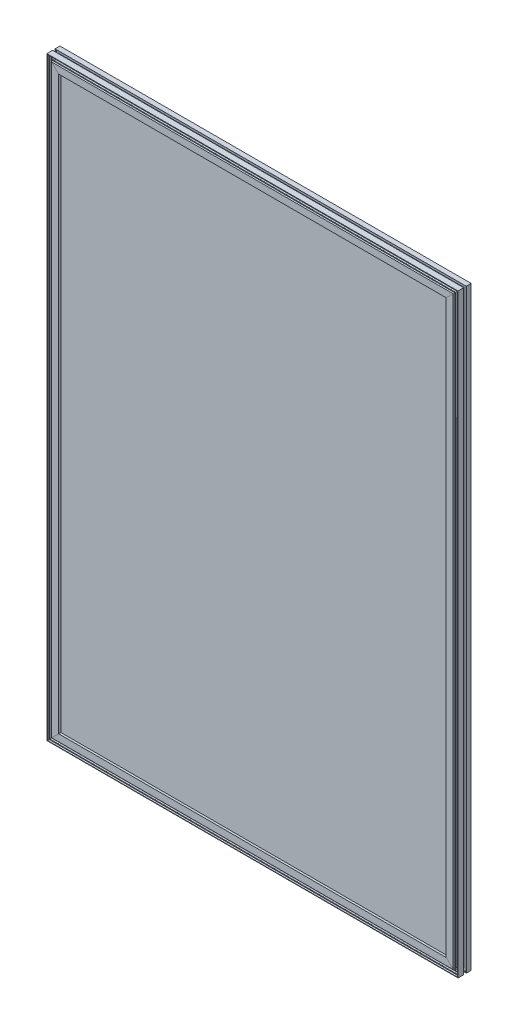
from build123d import *

# Parameters (mm, degrees)
MEMBER_250403_1_DEPTH      = 41.360872141
MEMBER_250403_1_DEPTH_BACK = 1401.360872141
MEMBER_250403_1_2_DEPTH    = 1022.721744282
MEMBER_250403_1_3_DEPTH    = 1442.721744282
MEMBER_250403_1_4_DEPTH    = 1022.721744282
SKETCH_12_W                = 900
SKETCH_12_H                = 1320
EXTRUDE_1_DEPTH            = 17


with BuildPart() as part:
    # 草图11 → Member 250403_1 (new, two sides: drawn at the far end of the back side and taken through both)
    with BuildSketch(Plane(origin=(-470, 680, 0), x_dir=(1, 0, 0), z_dir=(0, 1, 0)).offset(-MEMBER_250403_1_DEPTH_BACK)):
        with BuildLine():
            Line((11.006838108, 0), (27, 0))
            Line((27, 0), (27, 5))
            Line((27, 5), (25.5, 5))
            Line((25.5, 5), (25.5, 2.2))
            ThreePointArc((25.5, 2.2), (25.207106781, 1.492893219), (24.5, 1.2))
            Line((24.5, 1.2), (18, 1.2))
            ThreePointArc((18, 1.2), (17.292893219, 1.492893219), (17, 2.2))
            Line((17, 2.2), (17, 30))
            Line((17, 30), (12.5, 30))
            Line((12.5, 30), (12.5, 28.8))
            Line((12.5, 28.8), (15.8, 28.8))
            Line((15.8, 28.8), (15.8, 22))
            Line((15.8, 22), (1.2, 22))
            Line((1.2, 22), (1.2, 28.8))
            Line((1.2, 28.8), (4.5, 28.8))
            Line((4.5, 28.8), (4.5, 30))
            Line((4.5, 30), (0, 30))
            Line((0, 30), (0, 18.8))
            Line((0, 18.8), (1.2, 18.8))
            Line((1.2, 18.8), (1.2, 20.8))
            Line((1.2, 20.8), (6.7, 20.8))
            Line((6.7, 20.8), (6.7, 18.8))
            Line((6.7, 18.8), (7.7, 18.8))
            Line((7.7, 18.8), (7.7, 13))
            Line((7.7, 13), (6.7, 13))
            Line((6.7, 13), (6.7, 11))
            Line((6.7, 11), (1.2, 11))
            Line((1.2, 11), (1.2, 13))
            Line((1.2, 13), (0, 13))
            Line((0, 13), (0, 0))
            Line((0, 0), (1.006838108, 0))
            Line((1.006838108, 0), (2.380431303, 2.400675266))
            ThreePointArc((2.380431303, 2.400675266), (2.379848147, 2.600337065), (2.206838108, 2.7))
            Line((2.206838108, 2.7), (1.706838108, 2.7))
            Line((1.706838108, 2.7), (1.706838108, 2.9))
            Line((1.706838108, 2.9), (2.675186721, 3.252126768))
            ThreePointArc((2.675186721, 3.252126768), (2.770651604, 3.325346014), (2.806838108, 3.440085453))
            Line((2.806838108, 3.440085453), (2.806838108, 3.9))
            ThreePointArc((2.806838108, 3.9), (2.748259465, 4.041421356), (2.606838108, 4.1))
            Line((2.606838108, 4.1), (1.006838108, 4.1))
            Line((1.006838108, 4.1), (1.006838108, 9.5))
            ThreePointArc((1.006838108, 9.5), (1.153284718, 9.853553391), (1.506838108, 10))
            Line((1.506838108, 10), (10.506838108, 10))
            ThreePointArc((10.506838108, 10), (10.860391499, 9.853553391), (11.006838108, 9.5))
            Line((11.006838108, 9.5), (11.006838108, 4.1))
            Line((11.006838108, 4.1), (9.406838108, 4.1))
            ThreePointArc((9.406838108, 4.1), (9.265416752, 4.041421356), (9.206838108, 3.9))
            Line((9.206838108, 3.9), (9.206838108, 3.440085453))
            ThreePointArc((9.206838108, 3.440085453), (9.243024613, 3.325346014), (9.338489496, 3.252126768))
            Line((9.338489496, 3.252126768), (10.306838108, 2.9))
            Line((10.306838108, 2.9), (10.306838108, 2.7))
            Line((10.306838108, 2.7), (9.806838108, 2.7))
            ThreePointArc((9.806838108, 2.7), (9.63382807, 2.600337065), (9.633244913, 2.400675266))
            Line((9.633244913, 2.400675266), (11.006838108, 0))
        make_face()
        with BuildLine():
            Line((7.9, 11), (7.9, 11.8))
            ThreePointArc((7.9, 11.8), (8.607106781, 12.092893219), (8.9, 12.8))
            Line((8.9, 12.8), (8.9, 19))
            ThreePointArc((8.9, 19), (8.607106781, 19.707106781), (7.9, 20))
            Line((7.9, 20), (7.9, 20.8))
            Line((7.9, 20.8), (16, 20.8))
            Line((16, 20.8), (16, 1.2))
            Line((16, 1.2), (12.006838108, 1.2))
            Line((12.006838108, 1.2), (12.006838108, 11))
            Line((12.006838108, 11), (7.9, 11))
        make_face(mode=Mode.SUBTRACT)
    extrude(amount=MEMBER_250403_1_DEPTH + MEMBER_250403_1_DEPTH_BACK)

    # Member 250403_1 mitre 1
    split(bisect_by=Plane(origin=(-470, 680, 0), x_dir=(0.707106781, -0.707106781, 0), z_dir=(-0.707106781, -0.707106781, 0)), keep=Keep.TOP)

    # Member 250403_1 mitre 2
    split(bisect_by=Plane(origin=(-470, -680, 0), x_dir=(-0.707106781, -0.707106781, 0), z_dir=(-0.707106781, 0.707106781, 0)), keep=Keep.TOP)


with BuildPart() as body_2:
    # 草图11 on segment 2 (carried to segment 2) → Member 250403_1 2 (new body)
    with BuildSketch(Plane(origin=(511.360872141, -680, 0), x_dir=(0, 1, 0), z_dir=(-1, 0, 0))):
        with BuildLine():
            Line((11.006838108, 0), (27, 0))
            Line((27, 0), (27, 5))
            Line((27, 5), (25.5, 5))
            Line((25.5, 5), (25.5, 2.2))
            ThreePointArc((25.5, 2.2), (25.207106781, 1.492893219), (24.5, 1.2))
            Line((24.5, 1.2), (18, 1.2))
            ThreePointArc((18, 1.2), (17.292893219, 1.492893219), (17, 2.2))
            Line((17, 2.2), (17, 30))
            Line((17, 30), (12.5, 30))
            Line((12.5, 30), (12.5, 28.8))
            Line((12.5, 28.8), (15.8, 28.8))
            Line((15.8, 28.8), (15.8, 22))
            Line((15.8, 22), (1.2, 22))
            Line((1.2, 22), (1.2, 28.8))
            Line((1.2, 28.8), (4.5, 28.8))
            Line((4.5, 28.8), (4.5, 30))
            Line((4.5, 30), (0, 30))
            Line((0, 30), (0, 18.8))
            Line((0, 18.8), (1.2, 18.8))
            Line((1.2, 18.8), (1.2, 20.8))
            Line((1.2, 20.8), (6.7, 20.8))
            Line((6.7, 20.8), (6.7, 18.8))
            Line((6.7, 18.8), (7.7, 18.8))
            Line((7.7, 18.8), (7.7, 13))
            Line((7.7, 13), (6.7, 13))
            Line((6.7, 13), (6.7, 11))
            Line((6.7, 11), (1.2, 11))
            Line((1.2, 11), (1.2, 13))
            Line((1.2, 13), (0, 13))
            Line((0, 13), (0, 0))
            Line((0, 0), (1.006838108, 0))
            Line((1.006838108, 0), (2.380431303, 2.400675266))
            ThreePointArc((2.380431303, 2.400675266), (2.379848147, 2.600337065), (2.206838108, 2.7))
            Line((2.206838108, 2.7), (1.706838108, 2.7))
            Line((1.706838108, 2.7), (1.706838108, 2.9))
            Line((1.706838108, 2.9), (2.675186721, 3.252126768))
            ThreePointArc((2.675186721, 3.252126768), (2.770651604, 3.325346014), (2.806838108, 3.440085453))
            Line((2.806838108, 3.440085453), (2.806838108, 3.9))
            ThreePointArc((2.806838108, 3.9), (2.748259465, 4.041421356), (2.606838108, 4.1))
            Line((2.606838108, 4.1), (1.006838108, 4.1))
            Line((1.006838108, 4.1), (1.006838108, 9.5))
            ThreePointArc((1.006838108, 9.5), (1.153284718, 9.853553391), (1.506838108, 10))
            Line((1.506838108, 10), (10.506838108, 10))
            ThreePointArc((10.506838108, 10), (10.860391499, 9.853553391), (11.006838108, 9.5))
            Line((11.006838108, 9.5), (11.006838108, 4.1))
            Line((11.006838108, 4.1), (9.406838108, 4.1))
            ThreePointArc((9.406838108, 4.1), (9.265416752, 4.041421356), (9.206838108, 3.9))
            Line((9.206838108, 3.9), (9.206838108, 3.440085453))
            ThreePointArc((9.206838108, 3.440085453), (9.243024613, 3.325346014), (9.338489496, 3.252126768))
            Line((9.338489496, 3.252126768), (10.306838108, 2.9))
            Line((10.306838108, 2.9), (10.306838108, 2.7))
            Line((10.306838108, 2.7), (9.806838108, 2.7))
            ThreePointArc((9.806838108, 2.7), (9.63382807, 2.600337065), (9.633244913, 2.400675266))
            Line((9.633244913, 2.400675266), (11.006838108, 0))
        make_face()
        with BuildLine():
            Line((7.9, 11), (7.9, 11.8))
            ThreePointArc((7.9, 11.8), (8.607106781, 12.092893219), (8.9, 12.8))
            Line((8.9, 12.8), (8.9, 19))
            ThreePointArc((8.9, 19), (8.607106781, 19.707106781), (7.9, 20))
            Line((7.9, 20), (7.9, 20.8))
            Line((7.9, 20.8), (16, 20.8))
            Line((16, 20.8), (16, 1.2))
            Line((16, 1.2), (12.006838108, 1.2))
            Line((12.006838108, 1.2), (12.006838108, 11))
            Line((12.006838108, 11), (7.9, 11))
        make_face(mode=Mode.SUBTRACT)
    extrude(amount=MEMBER_250403_1_2_DEPTH)

    # Member 250403_1 2 mitre 1
    split(bisect_by=Plane(origin=(-470, -680, 0), x_dir=(0.707106781, 0.707106781, 0), z_dir=(0.707106781, -0.707106781, 0)), keep=Keep.TOP)

    # Member 250403_1 2 mitre 2
    split(bisect_by=Plane(origin=(470, -680, 0), x_dir=(0.707106781, -0.707106781, 0), z_dir=(-0.707106781, -0.707106781, 0)), keep=Keep.TOP)


with BuildPart() as body_3:
    # 草图11 on segment 3 (carried to segment 3) → Member 250403_1 3 (new body)
    with BuildSketch(Plane(origin=(470, 721.360872141, 0), x_dir=(-1, 0, 0), z_dir=(0, -1, 0))):
        with BuildLine():
            Line((11.006838108, 0), (27, 0))
            Line((27, 0), (27, 5))
            Line((27, 5), (25.5, 5))
            Line((25.5, 5), (25.5, 2.2))
            ThreePointArc((25.5, 2.2), (25.207106781, 1.492893219), (24.5, 1.2))
            Line((24.5, 1.2), (18, 1.2))
            ThreePointArc((18, 1.2), (17.292893219, 1.492893219), (17, 2.2))
            Line((17, 2.2), (17, 30))
            Line((17, 30), (12.5, 30))
            Line((12.5, 30), (12.5, 28.8))
            Line((12.5, 28.8), (15.8, 28.8))
            Line((15.8, 28.8), (15.8, 22))
            Line((15.8, 22), (1.2, 22))
            Line((1.2, 22), (1.2, 28.8))
            Line((1.2, 28.8), (4.5, 28.8))
            Line((4.5, 28.8), (4.5, 30))
            Line((4.5, 30), (0, 30))
            Line((0, 30), (0, 18.8))
            Line((0, 18.8), (1.2, 18.8))
            Line((1.2, 18.8), (1.2, 20.8))
            Line((1.2, 20.8), (6.7, 20.8))
            Line((6.7, 20.8), (6.7, 18.8))
            Line((6.7, 18.8), (7.7, 18.8))
            Line((7.7, 18.8), (7.7, 13))
            Line((7.7, 13), (6.7, 13))
            Line((6.7, 13), (6.7, 11))
            Line((6.7, 11), (1.2, 11))
            Line((1.2, 11), (1.2, 13))
            Line((1.2, 13), (0, 13))
            Line((0, 13), (0, 0))
            Line((0, 0), (1.006838108, 0))
            Line((1.006838108, 0), (2.380431303, 2.400675266))
            ThreePointArc((2.380431303, 2.400675266), (2.379848147, 2.600337065), (2.206838108, 2.7))
            Line((2.206838108, 2.7), (1.706838108, 2.7))
            Line((1.706838108, 2.7), (1.706838108, 2.9))
            Line((1.706838108, 2.9), (2.675186721, 3.252126768))
            ThreePointArc((2.675186721, 3.252126768), (2.770651604, 3.325346014), (2.806838108, 3.440085453))
            Line((2.806838108, 3.440085453), (2.806838108, 3.9))
            ThreePointArc((2.806838108, 3.9), (2.748259465, 4.041421356), (2.606838108, 4.1))
            Line((2.606838108, 4.1), (1.006838108, 4.1))
            Line((1.006838108, 4.1), (1.006838108, 9.5))
            ThreePointArc((1.006838108, 9.5), (1.153284718, 9.853553391), (1.506838108, 10))
            Line((1.506838108, 10), (10.506838108, 10))
            ThreePointArc((10.506838108, 10), (10.860391499, 9.853553391), (11.006838108, 9.5))
            Line((11.006838108, 9.5), (11.006838108, 4.1))
            Line((11.006838108, 4.1), (9.406838108, 4.1))
            ThreePointArc((9.406838108, 4.1), (9.265416752, 4.041421356), (9.206838108, 3.9))
            Line((9.206838108, 3.9), (9.206838108, 3.440085453))
            ThreePointArc((9.206838108, 3.440085453), (9.243024613, 3.325346014), (9.338489496, 3.252126768))
            Line((9.338489496, 3.252126768), (10.306838108, 2.9))
            Line((10.306838108, 2.9), (10.306838108, 2.7))
            Line((10.306838108, 2.7), (9.806838108, 2.7))
            ThreePointArc((9.806838108, 2.7), (9.63382807, 2.600337065), (9.633244913, 2.400675266))
            Line((9.633244913, 2.400675266), (11.006838108, 0))
        make_face()
        with BuildLine():
            Line((7.9, 11), (7.9, 11.8))
            ThreePointArc((7.9, 11.8), (8.607106781, 12.092893219), (8.9, 12.8))
            Line((8.9, 12.8), (8.9, 19))
            ThreePointArc((8.9, 19), (8.607106781, 19.707106781), (7.9, 20))
            Line((7.9, 20), (7.9, 20.8))
            Line((7.9, 20.8), (16, 20.8))
            Line((16, 20.8), (16, 1.2))
            Line((16, 1.2), (12.006838108, 1.2))
            Line((12.006838108, 1.2), (12.006838108, 11))
            Line((12.006838108, 11), (7.9, 11))
        make_face(mode=Mode.SUBTRACT)
    extrude(amount=MEMBER_250403_1_3_DEPTH)

    # Member 250403_1 3 mitre 1
    split(bisect_by=Plane(origin=(470, 680, 0), x_dir=(0.707106781, 0.707106781, 0), z_dir=(0.707106781, -0.707106781, 0)), keep=Keep.TOP)

    # Member 250403_1 3 mitre 2
    split(bisect_by=Plane(origin=(470, -680, 0), x_dir=(-0.707106781, 0.707106781, 0), z_dir=(0.707106781, 0.707106781, 0)), keep=Keep.TOP)


with BuildPart() as body_4:
    # 草图11 on segment 4 (carried to segment 4) → Member 250403_1 4 (new body)
    with BuildSketch(Plane(origin=(-511.360872141, 680, 0), x_dir=(0, -1, 0), z_dir=(1, 0, 0))):
        with BuildLine():
            Line((11.006838108, 0), (27, 0))
            Line((27, 0), (27, 5))
            Line((27, 5), (25.5, 5))
            Line((25.5, 5), (25.5, 2.2))
            ThreePointArc((25.5, 2.2), (25.207106781, 1.492893219), (24.5, 1.2))
            Line((24.5, 1.2), (18, 1.2))
            ThreePointArc((18, 1.2), (17.292893219, 1.492893219), (17, 2.2))
            Line((17, 2.2), (17, 30))
            Line((17, 30), (12.5, 30))
            Line((12.5, 30), (12.5, 28.8))
            Line((12.5, 28.8), (15.8, 28.8))
            Line((15.8, 28.8), (15.8, 22))
            Line((15.8, 22), (1.2, 22))
            Line((1.2, 22), (1.2, 28.8))
            Line((1.2, 28.8), (4.5, 28.8))
            Line((4.5, 28.8), (4.5, 30))
            Line((4.5, 30), (0, 30))
            Line((0, 30), (0, 18.8))
            Line((0, 18.8), (1.2, 18.8))
            Line((1.2, 18.8), (1.2, 20.8))
            Line((1.2, 20.8), (6.7, 20.8))
            Line((6.7, 20.8), (6.7, 18.8))
            Line((6.7, 18.8), (7.7, 18.8))
            Line((7.7, 18.8), (7.7, 13))
            Line((7.7, 13), (6.7, 13))
            Line((6.7, 13), (6.7, 11))
            Line((6.7, 11), (1.2, 11))
            Line((1.2, 11), (1.2, 13))
            Line((1.2, 13), (0, 13))
            Line((0, 13), (0, 0))
            Line((0, 0), (1.006838108, 0))
            Line((1.006838108, 0), (2.380431303, 2.400675266))
            ThreePointArc((2.380431303, 2.400675266), (2.379848147, 2.600337065), (2.206838108, 2.7))
            Line((2.206838108, 2.7), (1.706838108, 2.7))
            Line((1.706838108, 2.7), (1.706838108, 2.9))
            Line((1.706838108, 2.9), (2.675186721, 3.252126768))
            ThreePointArc((2.675186721, 3.252126768), (2.770651604, 3.325346014), (2.806838108, 3.440085453))
            Line((2.806838108, 3.440085453), (2.806838108, 3.9))
            ThreePointArc((2.806838108, 3.9), (2.748259465, 4.041421356), (2.606838108, 4.1))
            Line((2.606838108, 4.1), (1.006838108, 4.1))
            Line((1.006838108, 4.1), (1.006838108, 9.5))
            ThreePointArc((1.006838108, 9.5), (1.153284718, 9.853553391), (1.506838108, 10))
            Line((1.506838108, 10), (10.506838108, 10))
            ThreePointArc((10.506838108, 10), (10.860391499, 9.853553391), (11.006838108, 9.5))
            Line((11.006838108, 9.5), (11.006838108, 4.1))
            Line((11.006838108, 4.1), (9.406838108, 4.1))
            ThreePointArc((9.406838108, 4.1), (9.265416752, 4.041421356), (9.206838108, 3.9))
            Line((9.206838108, 3.9), (9.206838108, 3.440085453))
            ThreePointArc((9.206838108, 3.440085453), (9.243024613, 3.325346014), (9.338489496, 3.252126768))
            Line((9.338489496, 3.252126768), (10.306838108, 2.9))
            Line((10.306838108, 2.9), (10.306838108, 2.7))
            Line((10.306838108, 2.7), (9.806838108, 2.7))
            ThreePointArc((9.806838108, 2.7), (9.63382807, 2.600337065), (9.633244913, 2.400675266))
            Line((9.633244913, 2.400675266), (11.006838108, 0))
        make_face()
        with BuildLine():
            Line((7.9, 11), (7.9, 11.8))
            ThreePointArc((7.9, 11.8), (8.607106781, 12.092893219), (8.9, 12.8))
            Line((8.9, 12.8), (8.9, 19))
            ThreePointArc((8.9, 19), (8.607106781, 19.707106781), (7.9, 20))
            Line((7.9, 20), (7.9, 20.8))
            Line((7.9, 20.8), (16, 20.8))
            Line((16, 20.8), (16, 1.2))
            Line((16, 1.2), (12.006838108, 1.2))
            Line((12.006838108, 1.2), (12.006838108, 11))
            Line((12.006838108, 11), (7.9, 11))
        make_face(mode=Mode.SUBTRACT)
    extrude(amount=MEMBER_250403_1_4_DEPTH)

    # Member 250403_1 4 mitre 1
    split(bisect_by=Plane(origin=(-470, 680, 0), x_dir=(-0.707106781, 0.707106781, 0), z_dir=(0.707106781, 0.707106781, 0)), keep=Keep.TOP)

    # Member 250403_1 4 mitre 2
    split(bisect_by=Plane(origin=(470, 680, 0), x_dir=(-0.707106781, -0.707106781, 0), z_dir=(-0.707106781, 0.707106781, 0)), keep=Keep.TOP)


with BuildPart() as body_5:
    # 草图12 → 凸台-拉伸1 (new body)
    with BuildSketch(Plane(origin=(0, 0, -5), x_dir=(-1, 0, 0), z_dir=(0, 0, -1))):
        Rectangle(SKETCH_12_W, SKETCH_12_H)
    extrude(amount=EXTRUDE_1_DEPTH)


solid = Compound([part.part, body_2.part, body_3.part, body_4.part, body_5.part])
